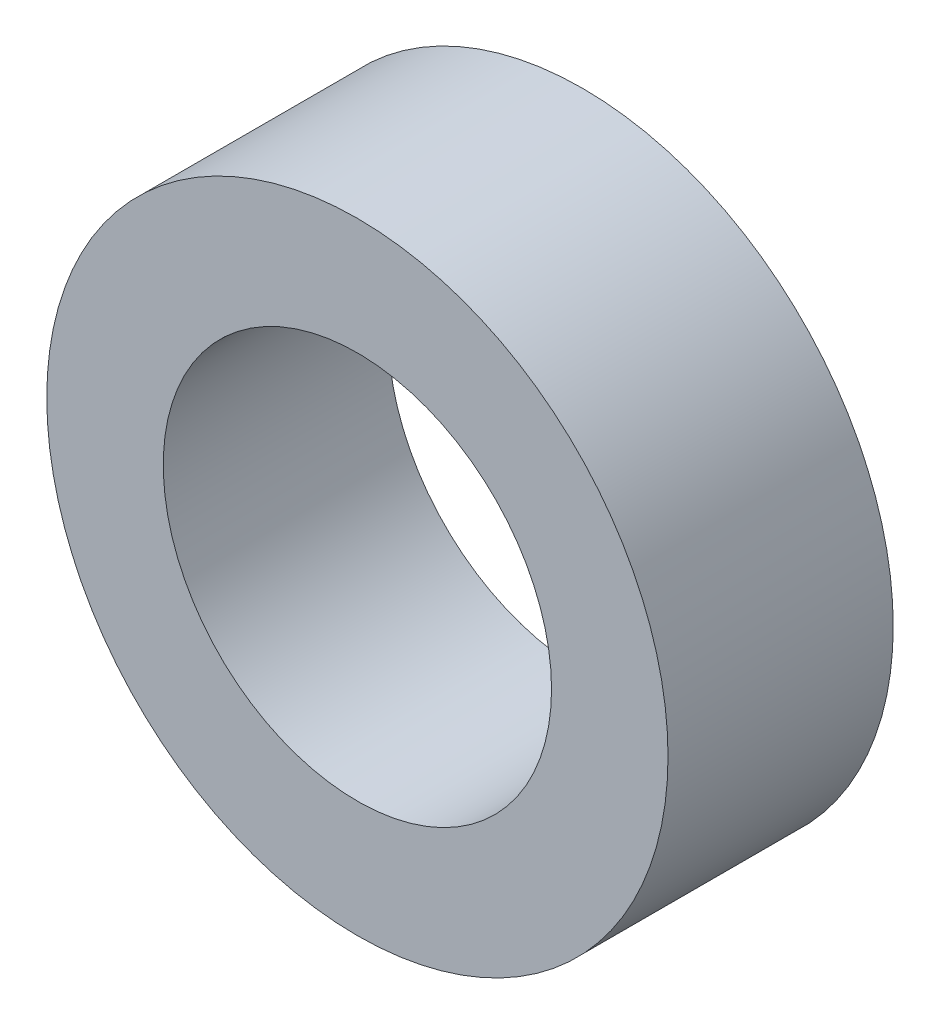
SolidWorks part; units mm, degrees
ref_plane "Front Plane" through (0, 0, 0) normal (0, 0, 1) x (1, 0, 0)
ref_plane "Top Plane" through (0, 0, 0) normal (0, 1, 0) x (1, 0, 0)
ref_plane "Right Plane" through (0, 0, 0) normal (1, 0, 0) x (0, 0, -1)
sketch "Sketch1" plane through (0, 0, 0) normal (0, 0, 1) x (1, 0, 0)
  circle A0 centre (0, 0) radius 2.5
  circle A1 centre (0, 0) radius 4
extrude "Boss-Extrude1" add sketch "Sketch1" along normal blind 2.9
